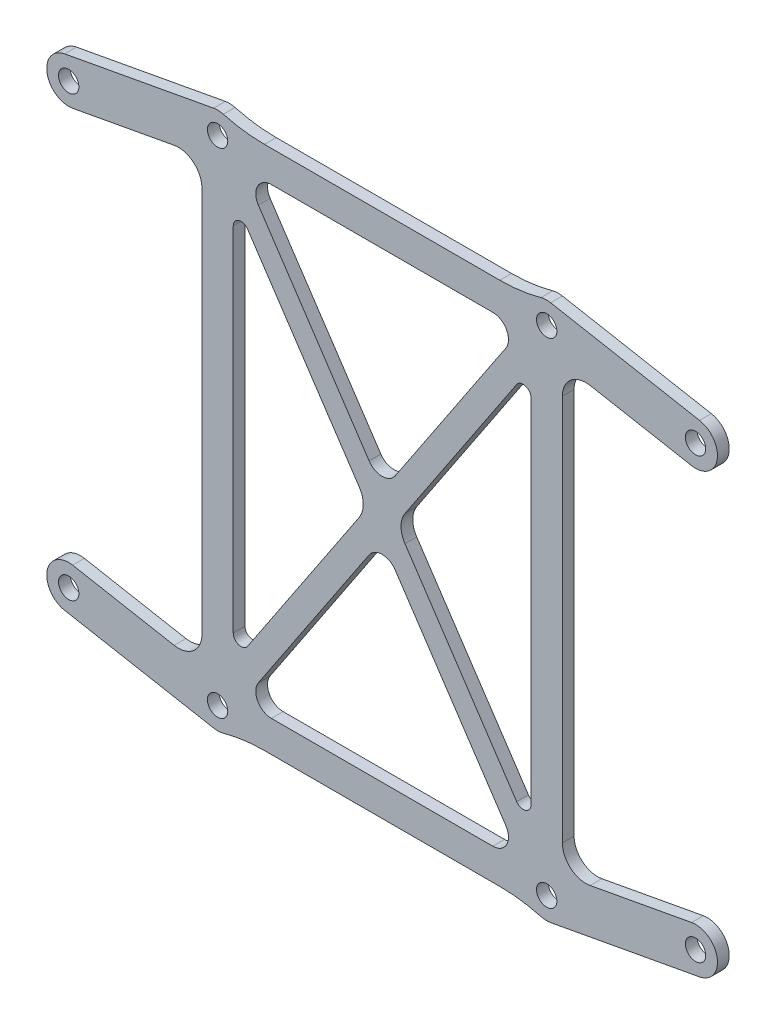
SolidWorks part; units mm, degrees
material "Thornel Mat VMA"
ref_plane "前视基准面" through (0, 0, 0) normal (0, 0, 1) x (1, 0, 0)
ref_plane "上视基准面" through (0, 0, 0) normal (0, 1, 0) x (1, 0, 0)
ref_plane "右视基准面" through (0, 0, 0) normal (1, 0, 0) x (0, 0, -1)
other "Configuration Table"
sketch "草图1" plane through (0, 0, 0) normal (0, 0, 1) x (1, 0, 0)
  line L0 (0, 0) -> (112.0484, 0) construction
  line L1 (-21, 31.5) -> (21, 31.5) construction
  line L2 (-21, 31.5) -> (-21, -31.5) construction
  line L3 (-21, -31.5) -> (21, -31.5) construction
  line L4 (21, 31.5) -> (21, -31.5) construction
  line L5 (-21, 31.5) -> (21, -31.5) construction
  line L6 (-21, -31.5) -> (21, 31.5) construction
  line L7 (0, 0) -> (0, 68.6393) construction
  line L8 (36, 87.8045) -> (36, -69.4668) construction
  line L9 (44, 87.8045) -> (44, -69.4668) construction
  line L10 (-44, 87.8045) -> (-44, -69.4668) construction
  line L11 (-36, 87.8045) -> (-36, -69.4668) construction
  line L12 (40, 0) -> (40, 28) construction
  line L13 (-40, 28) -> (-21, 31.5) construction
  line L14 (-40.5073, 30.7537) -> (-21.5073, 34.2537)
  line L15 (-39.4927, 25.2463) -> (-20.4927, 28.7463)
  line L16 (-21, 31.5) -> (21, 31.5) construction
  line L17 (-21, 33.5) -> (21, 33.5)
  line L18 (-21, 29.5) -> (21, 29.5)
  line L19 (-21, 31.5) -> (-21, -31.5) construction
  line L20 (-19, 31.5) -> (-19, -31.5)
  line L21 (-23, 31.5) -> (-23, -31.5)
  line L22 (-21, -31.5) -> (21, -31.5) construction
  line L23 (-21, -29.5) -> (21, -29.5)
  line L24 (-21, -33.5) -> (21, -33.5)
  line L25 (21, 31.5) -> (21, -31.5) construction
  line L26 (23, 31.5) -> (23, -31.5)
  line L27 (19, 31.5) -> (19, -31.5)
  line L28 (-21, 31.5) -> (21, -31.5) construction
  line L29 (-19.7519, 32.3321) -> (22.2481, -30.6679)
  line L30 (-22.2481, 30.6679) -> (19.7519, -32.3321)
  line L31 (-21, -31.5) -> (21, 31.5) construction
  line L32 (-22.2481, -30.6679) -> (19.7519, 32.3321)
  line L33 (-19.7519, -32.3321) -> (22.2481, 30.6679)
  line L34 (-40, -28) -> (-21, -31.5) construction
  line L35 (-39.4927, -25.2463) -> (-20.4927, -28.7463)
  line L36 (-40.5073, -30.7537) -> (-21.5073, -34.2537)
  line L37 (40, -28) -> (21, -31.5) construction
  line L38 (39.4927, -25.2463) -> (20.4927, -28.7463)
  line L39 (40.5073, -30.7537) -> (21.5073, -34.2537)
  line L40 (40, 28) -> (21, 31.5) construction
  line L41 (40.5073, 30.7537) -> (21.5073, 34.2537)
  line L42 (39.4927, 25.2463) -> (20.4927, 28.7463)
  circle A0 centre (21, 31.5) radius 1.3
  circle A1 centre (21, -31.5) radius 1.3
  circle A2 centre (-21, -31.5) radius 1.3
  circle A3 centre (-21, 31.5) radius 1.3
  circle A4 centre (40, 28) radius 1.3
  circle A5 centre (40, -28) radius 1.3
  circle A6 centre (-40, 28) radius 1.3
  circle A7 centre (-40, -28) radius 1.3
  arc A8 (-40.5073, 30.7537) -> (-39.4927, 25.2463) centre (-40, 28) ccw
  arc A9 (-20.4927, 28.7463) -> (-21.5073, 34.2537) centre (-21, 31.5) ccw
  arc A10 (-21, 33.5) -> (-21, 29.5) centre (-21, 31.5) ccw
  arc A11 (21, 29.5) -> (21, 33.5) centre (21, 31.5) ccw
  arc A12 (-19, 31.5) -> (-23, 31.5) centre (-21, 31.5) ccw
  arc A13 (-23, -31.5) -> (-19, -31.5) centre (-21, -31.5) ccw
  arc A14 (-21, -29.5) -> (-21, -33.5) centre (-21, -31.5) ccw
  arc A15 (21, -33.5) -> (21, -29.5) centre (21, -31.5) ccw
  arc A16 (23, 31.5) -> (19, 31.5) centre (21, 31.5) ccw
  arc A17 (19, -31.5) -> (23, -31.5) centre (21, -31.5) ccw
  arc A18 (-19.7519, 32.3321) -> (-22.2481, 30.6679) centre (-21, 31.5) ccw
  arc A19 (19.7519, -32.3321) -> (22.2481, -30.6679) centre (21, -31.5) ccw
  arc A20 (-22.2481, -30.6679) -> (-19.7519, -32.3321) centre (-21, -31.5) ccw
  arc A21 (22.2481, 30.6679) -> (19.7519, 32.3321) centre (21, 31.5) ccw
  arc A22 (-39.4927, -25.2463) -> (-40.5073, -30.7537) centre (-40, -28) ccw
  arc A23 (-21.5073, -34.2537) -> (-20.4927, -28.7463) centre (-21, -31.5) ccw
  arc A24 (39.4927, -25.2463) -> (40.5073, -30.7537) centre (40, -28) cw
  arc A25 (21.5073, -34.2537) -> (20.4927, -28.7463) centre (21, -31.5) cw
  arc A26 (40.5073, 30.7537) -> (39.4927, 25.2463) centre (40, 28) cw
  arc A27 (20.4927, 28.7463) -> (21.5073, 34.2537) centre (21, 31.5) cw
  point P0 (0, 0)
  point P24 (-30.5, 29.75)
  point P36 (0, 31.5)
  point P42 (-21, 0)
  point P48 (0, -31.5)
  point P55 (21, 0)
  point P62 (0, 0)
  point P69 (0, 0)
  point P74 (-30.5, -29.75)
  point P81 (30.5, -29.75)
  point P87 (30.5, 29.75)
  dimension "D3" = 2.6
  dimension "D7" = 2.6
  dimension "D8" = 28
  dimension "D9" = 1.5
  dimension "D10" = 2
  dimension "D11" = 2.8
  dimension "D1" = 63
  dimension "D2" = 42
  dimension "D4" = 8
  dimension "D5" = 72
  dimension "D6" = 4
extrude "凸台-拉伸1" add sketch "草图1" along normal blind 1.5 contours A10 L17 A9 L14 A8 L15 L21 A6 | A10 L21 L15 L30 | A10 L30 L15 A9 L18 | L20 A12 A10 L18 A9 A3 | A12 L29 A9 L17 | A12 L20 A9 L29 | A9 L20 L18 L29 | A9 L18 L20 | A9 L15 L30 L20 L18 | L21 L35 L32 L20 L30 L15 | L36 A23 L24 A13 L21 L35 A22 A7 | A14 L32 L35 L21 | L23 A23 L35 L32 A14 | L20 A23 L23 A14 A13 A2 | A23 L23 L20 L32 L35 | L23 L33 L30 L32 L20 | A23 L20 L23 | A23 L33 L23 L20 | L33 A23 L20 A13 | L24 A23 L33 A13 | L24 A25 L30 L23 L33 A23 | A25 L24 A17 L30 | A25 L39 A24 L38 L26 A15 L24 A5 | A25 L27 A17 A15 L23 A1 | A25 L23 A15 L29 L38 | L30 A25 L27 L23 | A25 L30 A17 L27 | L27 A25 L23 | L23 A25 L38 L29 L27 | L33 L30 L23 L27 L29 | A15 L26 L38 L29 | L26 L42 L33 L27 L29 L38 | L30 L33 L29 L32 | L30 L32 L29 L18 L20 | L29 L33 L27 L18 L32 | L32 A27 L17 A9 L29 L18 | L42 A27 L18 L27 L33 | L27 A27 L32 L18 | A27 L27 A16 L32 | L18 A27 L27 | A27 L32 A16 L17 | A27 L17 A11 L26 L42 A26 L41 A4 | A27 L18 A11 A16 L27 A0 | A27 L42 L33 A11 L18 | A11 L33 L42 L26 | L29 A18 L30 A10 L18 L20 A3 | L33 A21 L32 L27 L18 A11 A0 | L32 A20 L33 L20 L23 A14 A2 | L30 A19 L29 A15 L23 L27 A1
fillet "圆角1" radius 2 6 edges at (17.8639, -29.5, 0.75) (-17.8639, -29.5, 0.75) (0, -2.7042, 0.75) (0, 2.7042, 0.75) (17.8639, 29.5, 0.75) (-17.8639, 29.5, 0.75)
fillet "圆角2" radius 1 4 edges at (19, -25.7958, 0.75) (19, 25.7958, 0.75) (-19, -25.7958, 0.75) (-19, 25.7958, 0.75)
fillet "圆角3" radius 20 4 edges at (-19.0404, 33.5, 0.75) (19.0404, 33.5, 0.75) (19.0404, -33.5, 0.75) (-19.0404, -33.5, 0.75)
fillet "圆角4" radius 3 6 edges at (-1.8028, 0, 0.75) (1.8028, 0, 0.75) (23, 28.2845, 0.75) (23, -28.2845, 0.75) (-23, -28.2845, 0.75) (-23, 28.2845, 0.75)
